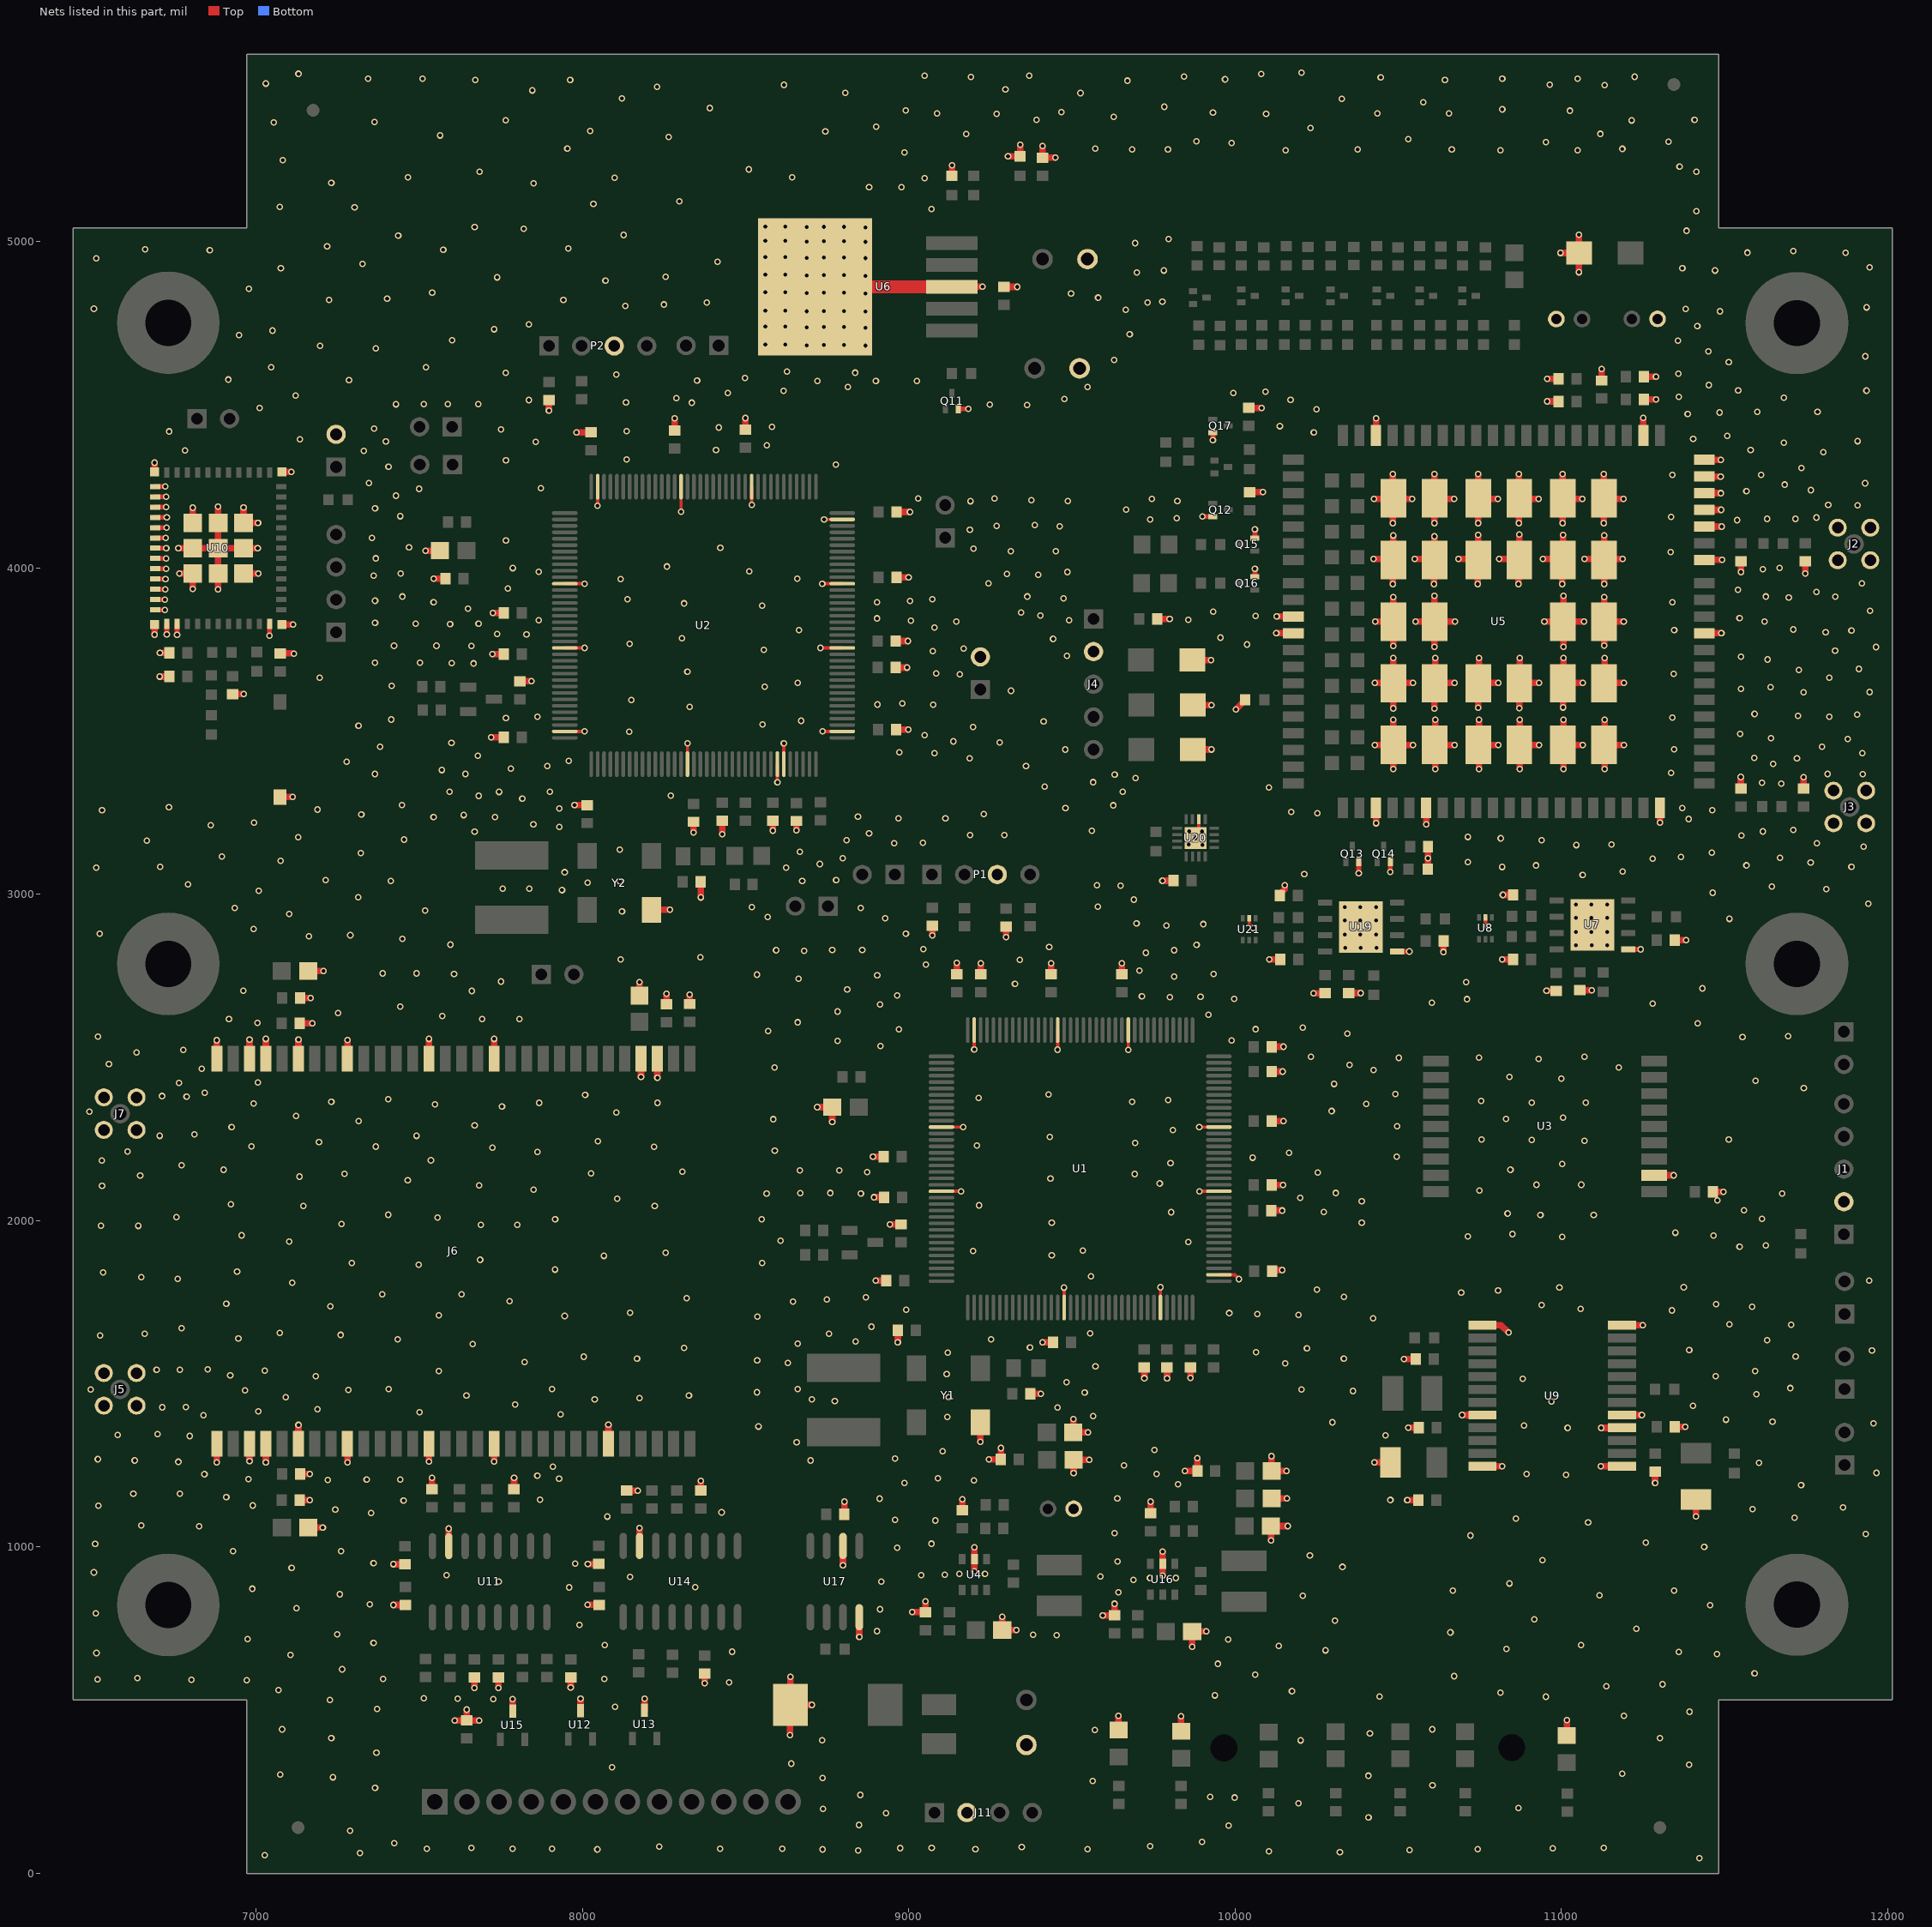
[diagram p0: the nets of this part, all layers, seen from the top]
# Altium PCB MISC86294.PcbDoc (part 4 of 8)
Units mil, origin at the board's own origin, x right, y up, seen from the top; angles counter-clockwise.
Board outline 5574.84 x 5574.84 mil, 4 copper layers (Top, GND02, PWR03, Bottom), stack 23.756 mil thick; 313 components, 311 nets, 1350 pads, 1701 vias.

## Via types
v1: diameter 20, hole 12, Top to Bottom, 1701 vias

## Nets (pads, with @x,y where several pads share a name; then routed paths per layer and width w, separated by ;. In a path a pad name is that pad's centre, name@x,y a point inside that pad or via, vN(x,y) a via of type N, cw(c..) or ccw(c..) an arc to the next point about the centre after c; other vN are vias at no path point) (continued)
GND: C1.1 C2.2 C3.2 C4.2 C5.2 C6.2 C7.2 C8.2 C9.2 C10.2 C11.2 C12.2 C13.2 C14.2 C15.2 C16.2 C17.2 C18.2 C19.1 C20.2 C21.2 C22.2 C23.2 C24.2 C25.2 C26.2 C27.2 C28.2 C29.2 C30.2 C31.2 C32.2 C33.2 C34.2 C35.2 C36.2 C37.2 C40.2 C41.2 C42.2 C43.2 C44.1 C45.1 C46.2 C49.2 C50.2 C51.2 C52.2 C53.1 C55.1 C56.1 C59.2 C60.2 C61.2 C62.2 C64.2 C65.2 C66.2 C67.2 C69.1 C70.1 C74.2 C75.2 C76.2 C77.2 C78.2 C79.2 C80.2 C81.2 C82.2 C83.2 C84.2 C85.2 C86.1 C87.2 C88.2 C89.1 C90.1 C91.1 C92.1 C93.2 C94.2 C95.2 C96.2 C97.2 C98.2 C99.1 C100.1 C101.1 C102.1 C103.1 C104.1 C105.2 C107.2 C110.2 C111.2 C112.2 C113.2 C115.1 C116.1 C117.2 C118.1 C119.1 C120.2 C121.2 C122.1 C123.2 C124.1 C128.2 C129.2 C130.2 C200.1 C201.2 C202.1 C203.2 D1.1 D2.2 D3.2 D4.1 D5.1 D6.1 D7.1 D11.2 J1.2 J2.2 J2.3 J2.4 J2.5 J3.2 J3.3 J3.4 J3.5 J4.2 J5.2 J5.3 J5.4 J5.5 J6.1 J6.3 J6.4 J6.6 J6.9 J6.14 J6.18 J6.25 J6.33 J6.34 J6.43 J6.47 J6.52 J6.55 J6.57 J6.58 J6.60 J7.2 J7.3 J7.4 J7.5 J9.2 J11.2 J23.2 L3.2 P1.3 P2.3 Q11.2 Q12.2 Q13.2 Q14.2 Q15.2 Q16.2 Q17.2 R3.1 R5.1 R11.2 R16.1 R18.1 R20.2 R28.1 R33.1 R61.1 R62.1 R63.1 R85.2 SW1.1 U1.16 U1.31 U1.38 U1.51 U1.61 U1.83 U1.94 U1.107 U1.120 U1.130 U2.16 U2.30 U2.31 U2.38 U2.51 U2.61 U2.71 U2.83 U2.94 U2.107 U2.120 U2.130 U2.143 U3.2 U4.2 U5.8 U5.9 U5.19 U5.22 U5.36 U5.46 U5.48 U5.50 U5.51 U5.52 U5.53 U5.54 U5.56 U5.72 U5.85 U5.86 U5.87 U5.88 U5.89 U5.90 U5.91 U5.92 U5.93 U5.94 U5.95 U5.96 U5.97 U5.98 U5.99 U5.100 U5.101 U5.102 U5.103 U5.104 U5.105 U5.106 U5.107 U5.108 U5.109 U5.110 U5.111 U5.112 U6.3 U6.6 U7.1 U7.9 U8.2 U9.1 U9.8 U9.12 U9.13 U9.16 U9.17 U9.24 U10.1 U10.2 U10.11 U10.36 U10.37 U10.38 U10.39 U10.40 U10.41 U10.42 U10.43 U10.44 U10.45 U10.46 U10.47 U10.48 U10.49 U10.50 U10.51 U10.52 U10.53 U11.15 U12.3 U13.3 U14.15 U15.3 U16.2 U17.2 U17.8 U19.1 U19.9 U20.6 U20.17 U21.2 Y1.2 Y2.2 | length 18190.1
  Top w10: U2.143@7945.42,3499.52 v1(8006.52,3499.52) ; U2.130@7945.42,3755.43 v1(8006.57,3755.43) ; U2.120@7945.42,3952.28 v1(8005.72,3952.28) ; v1(8045.81,4191.19) U2.107@8045.81,4249.52 ; v1(8301.71,4172.71) U2.94@8301.71,4249.52 ; U2.16@8321.4,3399.13 v1(8321.4,3462.6) ; v1(8518.25,4193.25) U2.83@8518.25,4249.52 ; v1(8596.99,3343.01) U2.30@8596.99,3399.13 ; U2.31@8616.67,3399.13 v1(8616.67,3463.32) ; v1(8728.57,3755.43) U2.51@8795.81,3755.43 ; v1(8734.72,3952.28) U2.61@8795.81,3952.28 ; v1(8735.52,3499.52) U2.38@8795.81,3499.52 ; v1(8740.13,4149.13) U2.71@8795.81,4149.13 ; U1.130@9099.8,2090.1 v1(9160.1,2090.1) ; U1.120@9099.8,2286.95 v1(9166.05,2286.95) ; v1(9200.2,2524.8) U1.107@9200.2,2584.2 ; v1(9456.1,2524.1) U1.94@9456.1,2584.2 ; U1.16@9475.79,1733.8 v1(9475.79,1794.79) ; v1(9672.64,2523.36) U1.83@9672.64,2584.2 ; U1.31@9771.06,1733.8 v1(9771.06,1795.94) ; U20.17@9888.99,3203.01 U20.6@9888.99,3230.12 ; v1(9890.05,2286.95) U1.61@9950.2,2286.95 ; v1(9891.1,2090.1) U1.51@9950.2,2090.1 ; U1.38@9950.2,1834.2 9998.8,1834.2 v1(10012,1821) ; U21.2@10043,2926.47 10043,2909 v1(10055,2897)
  Top w12: v1@10767,2909 U8.2@10767,2929.47 ; v1@10773,2904 10772.5,2903.5 10773.5,2903.5 10773.62,2903.62 v1(10774.3,2903.62)
  Top w15: U10.48@6690.09,3872.02 v1(6719.98,3872.02) ; U10.47@6690.09,3903.52 v1(6719.52,3903.52) ; U10.46@6690.09,3935.02 v1(6721.02,3935.02) ; U10.45@6690.09,3966.51 v1(6721.51,3966.51) ; U10.44@6690.09,3998.01 v1(6722.99,3998.01) ; U10.43@6690.09,4029.5 v1(6723.5,4029.5) ; U10.42@6690.09,4061 v1(6724,4061) ; U10.41@6690.09,4092.5 v1(6722.5,4092.5) ; U10.40@6690.09,4123.99 v1(6724.99,4123.99) ; U10.39@6690.09,4155.49 v1(6725.49,4155.49) ; U10.38@6690.09,4186.98 v1(6723.98,4186.98) ; U10.37@6690.09,4218.48 v1(6723.48,4218.48) ; U10.36@6690.09,4249.98 v1(6720.98,4249.98) ; v1(6725.52,3796.52) U10.1@6725.52,3828.72 ; v1(6757.02,3795.02) U10.2@6757.02,3828.72 ; v1(7040.48,3792.48) U10.11@7040.48,3828.72 ; Q11.2@9152.04,4487.7 v1(9182.3,4487.7) ; v1(9900.05,4158.05) Q12.2@9930.93,4158.05 ; v1(9931.93,4392.07) Q17.2@9931.93,4415.6 ; Q16.2@10060.74,3973.48 v1(10060.74,3998.26) ; Q15.2@10060.74,4092.48 v1(10060.74,4118.74) ; v1(10378.92,3065.08) Q13.2@10378.92,3099.74 ; v1(10475.68,3068.32) Q14.2@10475.68,3099.74 ; U19.1@10496.06,2825.03 v1(10534.03,2825.03) ; U7.1@11205.26,2831.5 v1(11242.5,2831.5)
  Top w20: v1(6688.12,3796.12) U10.53@6688.12,3826.75 ; U10.50@6688.12,4295.25 v1(6688.12,4323.12) ; v1(6703.54,3667.46) C102.1@6733.79,3667.46 ; v1(6704.46,3740.46) C103.1@6733.79,3740.46 ; v1(6760.99,4060.99) U10.49@6805.24,4060.99 ; v1(6764.24,3983.24) U10.49@6805.24,3983.24 v1(6805.24,3935.76) ; U10.49@6805.24,4138.75 v1(6805.24,4185.24) ; U10.49@6828.01,4060.99 U10.49@6883,4060.99 ; v1(6879.01,1258.99) J6.1@6879.01,1315.83 ; J6.60@6879.01,2496.94 v1(6879.01,2552.99) ; v1(6883,3935) U10.49@6883,3983.24 ; U10.49@6883,3998 U10.49@6883,4060.99 ; U10.49@6883,4113 U10.49@6883,4060.99 ; U10.49@6883,4138.75 v1(6883,4188) ; C104.1@6927.54,3613.79 v1(6961.79,3613.79) ; U10.49@6942.99,4060.99 U10.49@6883,4060.99 ; U10.49@6960.76,3983.24 v1(7006.24,3983.24) ; U10.49@6960.76,4060.99 v1(7003.99,4060.99) ; v1(6960.76,4185.76) U10.49@6960.76,4138.75 v1(7005.25,4138.75) ; v1(6979.01,1263.01) J6.3@6979.01,1315.83 ; J6.58@6979.01,2496.94 v1(6979.01,2555.01) ; v1(7029.01,1259.01) J6.4@7029.01,1315.83 ; J6.57@7029.01,2496.94 v1(7029.01,2557.01) ; SW1.1@7072.43,3298.37 v1(7111.37,3298.37) ; C105.2@7072.68,3738.82 v1@7113.18,3738.82 ; U10.52@7077.88,3826.75 v1(7112.75,3826.75) ; U10.51@7077.88,4295.25 v1(7106.75,4295.25) ; J6.6@7129.01,1315.83 v1(7129.01,1373.99) ; J6.55@7129.01,2496.94 v1(7129.01,2554.99) ; C90.1@7132.87,2604.56 v1(7171.56,2604.56) ; C88.2@7133.25,1143.3 v1(7163.7,1143.3) ; C87.2@7133.55,1223.2 v1(7163.8,1223.2) ; C89.1@7134.24,2682.56 v1(7166.56,2682.56) ; C91.1@7159.09,2765.45 v1(7205.55,2765.45) ; C86.1@7159.25,1059.3 v1(7203.7,1059.3) ; v1(7279.01,1259.01) J6.9@7279.01,1315.83 ; J6.52@7279.01,2496.94 v1(7279.01,2554.01) ; v1(7419.76,822.24) C110.2@7457.16,822.24 ; v1(7420.14,947.14) C107.2@7455.89,947.14 ; v1(7518.53,4053.47) C28.2@7562.55,4053.47 ; v1(7529.01,1262.01) J6.14@7529.01,1315.83 ; J6.47@7529.01,2496.94 v1(7529.01,2557.01) ; C115.1@7538.64,1177.45 v1(7538.64,1211.36) ; v1(7543.45,3967.55) C22.2@7579.14,3967.55 ; U11.15@7590.02,1002.38 v1(7590.02,1056.02) ; v1(7607.75,468.25) L3.2@7644.59,468.25 ; v1(7644.59,501.59) L3.2@7644.59,468.25 ; v1(7667.93,567.93) C113.2@7667.93,600.24 ; v1(7683.25,468.25) L3.2@7644.59,468.25 ; v1(7720,3481) C25.2@7758.14,3481 ; v1(7723.7,3736.7) C23.2@7758.14,3736.7 ; v1(7725.15,3862.85) C24.2@7758.14,3862.85 ; v1(7729.01,1261.99) J6.18@7729.01,1315.83 ; J6.43@7729.01,2496.94 v1(7729.01,2556.99) ; v1(7741.82,568.18) C121.2@7741.82,600.24 ; U15.3@7785.4,496.71 v1(7785.4,533.6) ; C116.1@7789.89,1177.45 v1(7789.89,1211.89) ; R16.1@7807.89,3653.25 v1(7843.25,3653.25) ; v1(7896.51,4482.51) R20.2@7896.51,4515.6 ; v1(7963.48,569.48) C120.2@7963.48,600.24 ; v1(7975.32,3273.68) C203.2@8014.05,3273.68 ; v1(7981.08,4415.92) C34.2@8026.08,4415.92 ; U12.3@7993.6,498.71 v1(7993.6,535.4) ; v1(8015.66,822.34) C112.2@8051.36,822.34 ; v1(8015.94,947.94) C111.2@8049.91,947.94 ; J6.25@8079.01,1315.83 v1(8079.01,1374.99) ; C118.1@8134.38,1172.45 v1(8169.55,1172.45) ; C101.1@8174.55,2690.09 v1(8174.55,2730.55) ; U14.15@8174.68,1003.16 v1(8174.68,1058.32) ; v1(8179.01,2440.99) J6.34@8179.01,2496.94 ; U13.3@8189.75,498.96 v1(8189.75,535.25) ; Y2.2@8209.69,2953.06 v1(8268.06,2953.06) ; v1(8229.01,2438.01) J6.33@8229.01,2496.94 ; C100.1@8257.44,2663.75 v1(8257.44,2695.56) ; C27.2@8281.83,4421.48 v1(8281.83,4459.17) ; C99.1@8328.44,2663.99 v1(8328.44,2692.44) ; v1(8339.7,3189.3) C29.2@8339.7,3222.52 ; C119.1@8361.88,1172.45 v1(8361.88,1202.88) ; v1(8362.29,2990.71) C202.1@8362.29,3026 ; v1(8374.53,582.53) C117.2@8374.53,612.24 ; v1(8428.25,3184.25) C19.1@8428.25,3224.63 ; C31.2@8498.76,4424.48 v1(8498.76,4459.77) ; v1(8582.6,3195.6) C21.2@8582.6,3226.14 ; v1(8636,423) D1.1@8636,465 ; v1(8636.87,602.13) D1.1@8636.87,516 v1(8703,516) ; v1(8655.74,3196.26) C20.2@8655.74,3225.14 ; v1(8719,2348) C12.2@8765.1,2348 v1(8765.1,2303.1) ; v1(8798,944) U17.2@8798,1003 ; C124.1@8802.11,1100.18 v1(8802.11,1138.89) ; v1(8848,724) U17.8@8848,784.7 ; v1(8889.94,2196.06) C14.2@8922.52,2196.06 ; v1(8893.17,2071.83) C13.2@8924.52,2071.83 ; v1(8898,1816) C11.2@8930.14,1816 ; v1(8941.5,1988.5) R3.1@8975.89,1988.5 ; R18.1@8959.03,3695.11 v1(8994.11,3695.11) ; C30.2@8959.48,3776.47 v1(8996.53,3776.47) ; C26.2@8960.48,3505.41 8997.59,3505.41 v1(8998,3505) ; C33.2@8961.77,4172.02 v1(9003.02,4172.02) ; C32.2@8962.48,3972 v1(8999,3972) ; v1(8965.99,1627.01) C201.2@8965.99,1664.16 ; v1(9010.25,800.25) C45.1@9050.89,800.25 v1(9050.89,832.89) ; v1(9071.89,2874.11) R11.2@9071.89,2903.92 ; U6.3@9132.07,4862.15 v1(9226.15,4862.15) ; R63.1@9132.17,5202.48 v1(9132.17,5234.83) ; C15.2@9147.3,2755.48 v1(9147.3,2790.3) ; R28.1@9163.89,1112.25 v1(9163.89,1145.89) ; v1(9201,925) U4.2@9201,962.24 v1(9201,999) ; v1(9219.62,1322.38) Y1.2@9219.62,1381.7 ; C2.2@9220.11,2755.48 v1(9220.11,2789.11) ; v1(9245.11,1268.11) C41.2@9282.14,1268.11 v1(9282.14,1303.14) ; v1(9286.2,785.8) C44.1@9286.2,745 v1(9329,745) ; C75.2@9291.05,4862.01 v1(9331.99,4862.01) ; v1(9298,2869) C1.1@9298,2901.75 ; v1(9303.84,5262.16) R61.1@9341.05,5262.16 v1(9341.05,5298.05) ; C200.1@9372.08,1469.16 v1(9404.16,1469.16) ; v1(9410,1627) C18.2@9441.52,1627 ; v1(9410.05,5293.95) C77.2@9410.05,5257.96 v1(9448.96,5257.96) ; C16.2@9435.53,2755.48 v1(9435.53,2788.53) ; v1(9503.9,1391.9) C40.2@9503.9,1351 v1(9549,1351) ; v1(9504.9,1226.1) C42.2@9504.9,1267 v1(9553,1267) ; v1(9594.32,790.32) C92.1@9630.01,790.32 v1(9630.01,825.99) ; D11.2@9642.55,438.8 v1(9642.55,482.45) ; C17.2@9652.76,2755.48 v1(9652.76,2788.76) ; v1(9721.74,1517.26) C6.2@9721.74,1550.14 ; R33.1@9740.89,1103.25 v1(9740.89,1138.89) ; C62.2@9760.83,3844.65 v1(9799.35,3844.65) ; v1(9777.11,3041.89) C122.1@9811.75,3041.89 ; v1(9778,912) U16.2@9778,948.24 v1(9778,986) ; v1(9791.37,1516.37) C5.2@9791.37,1550.14 ; D3.2@9834.55,434.8 v1(9834.55,481.55) ; v1(9846.11,1233.11) C50.2@9884.14,1233.11 v1(9884.14,1271.86) ; v1(9862.63,1518.37) C4.2@9862.63,1550.14 ; v1(9868.2,694.2) C53.1@9868.2,741 v1(9912,741) ; D5.1@9868.79,3718.07 v1(9926.07,3718.07) ; D6.1@9869.79,3444.07 v1(9927.93,3444.07) ; D7.1@9869.79,3580.07 v1(9927.93,3580.07) ; v1(10002,3567.34) R62.1@10030.74,3596.07 ; C81.2@10041.5,4490.93 v1(10080.93,4490.93) ; C78.2@10044.94,4232.93 v1(10084.93,4232.93) ; v1(10104.44,2800.56) C129.2@10138.47,2800.56 ; v1(10109.9,1020.1) C51.2@10109.9,1064 v1(10161,1064) ; R5.1@10111.25,2031.11 v1(10143.89,2031.11) ; C8.2@10111.86,2109.45 v1(10146.55,2109.45) ; C9.2@10111.86,2305.3 v1(10148.7,2305.3) ; C3.2@10111.86,2457 v1(10146,2457) ; C10.2@10111.86,2533.15 v1(10147.85,2533.15) ; C49.2@10111.9,1149 v1(10159,1149) ; v1(10111.9,1278.1) C52.2@10111.9,1233 v1(10157,1233) ; C7.2@10112.86,1848.6 v1(10144.4,1848.6) ; v1(10126.42,3800.57) U5.9@10178.08,3800.57 ; v1(10127.76,3851.76) U5.8@10178.08,3851.76 ; C123.2@10137.31,2996.24 10137.31,3001.31 10152,3016 v1(10152,3028) ; v1(10239.86,2697.14) C93.2@10275.89,2697.14 ; C128.2@10347.55,2697.47 v1(10384.53,2697.47) ; v1(10424.06,4027.94) 10483.84,4027.94 v1(10483.84,3951.16) ; v1(10425.94,4212.06) U5.108@10483.16,4212.06 ; v1(10427,1259) C37.2@10475.99,1259 ; v1(10427.94,3458.06) U5.112@10485.16,3458.06 ; v1(10427.94,3648.06) U5.111@10485.16,3648.06 ; v1(10429,3836.01) U5.110@10485.16,3836.01 ; v1(10432.01,3218.01) U5.19@10432.01,3265.13 ; U5.72@10432.01,4406.86 v1(10432.01,4458.99) ; v1(10483.16,4137.84) U5.108@10483.16,4212.06 ; v1(10483.16,4288.84) U5.108@10483.16,4212.06 ; v1(10485.16,3383.84) U5.112@10485.16,3458.06 ; v1(10485.16,3534.84) U5.112@10485.16,3458.06 ; v1(10485.16,3570.16) U5.111@10485.16,3647.02 ; v1(10485.16,3724.84) U5.111@10485.16,3648.06 ; v1(10485.16,3761.16) U5.110@10485.16,3836.01 ; v1(10485.16,3911.16) U5.110@10485.16,3836.01 ; U5.109@10485.16,4024.98 v1(10485.16,4099.84) ; v1(10517.89,1576.11) C96.2@10554.14,1576.11 ; v1(10527.5,1143.5) C98.2@10561.14,1143.5 ; v1(10530.98,1365.98) C94.2@10562.31,1365.98 ; v1(10542.94,4212.06) U5.108@10483.16,4212.06 ; v1(10544.94,3458.06) U5.112@10485.16,3458.06 ; v1(10544.94,3648.06) U5.111@10485.16,3648.06 ; v1(10550.06,4027.94) 10609.84,4027.94 v1(10609.84,3951.16) ; v1(10553,3836.01) U5.105@10611.15,3836.01 ; v1(10585.55,3214.55) U5.22@10585.55,3265.13 ; R85.2@10590.67,3077.13 v1@10590.67,3108.67 ; v1(10591.13,3110.87) C79.2@10591.13,3146.93 ; v1(10611.14,3569.86) U5.106@10611.14,3647.02 ; v1(10611.15,3759.15) U5.105@10611.15,3836.01 ; v1(10611.15,3914.85) U5.105@10611.15,3836.01 ; U5.104@10611.14,4024.98 v1(10611.14,4097.14) ; v1(10611.16,4137.84) U5.103@10611.16,4212.06 ; v1(10611.16,4288.84) U5.103@10611.16,4212.06 ; v1(10613.16,3383.84) U5.107@10613.16,3458.06 ; v1(10613.16,3534.84) U5.107@10613.16,3458.06 ; v1(10613.16,3724.84) 10613.16,3648.06 v1(10672.94,3648.06) ; v1(10638.53,2823.53) C130.2@10638.53,2856.97 ; v1(10670.94,4212.06) U5.103@10611.16,4212.06 ; v1(10672.94,3458.06) U5.107@10613.16,3458.06 ; v1(10674,3836.01) U5.105@10611.15,3836.01 ; v1(10684.06,4027.94) 10743.84,4027.94 v1(10743.84,3951.16) ; v1(10695.64,1404.36) U9.8@10758.02,1404.36 ; v1(10745,3572) U5.101@10745,3647.02 ; U5.100@10745,4024.98 v1(10745,4102) ; v1(10745.16,4137.84) U5.99@10745.16,4212.06 ; v1(10745.16,4288.84) U5.99@10745.16,4212.06 ; v1(10747.16,3383.84) U5.102@10747.16,3458.06 ; v1(10747.16,3534.84) U5.102@10747.16,3458.06 ; v1(10747.16,3724.84) 10747.16,3648.06 v1(10806.94,3648.06) ; U9.12@10758.02,1246.88 v1(10818.12,1246.88) ; U9.1@10758.02,1679.95 10815.05,1679.95 v1(10838,1657) ; v1(10804.94,4212.06) U5.99@10745.16,4212.06 ; v1(10806.94,3458.06) U5.102@10747.16,3458.06 ; v1(10809.06,4027.94) 10868.84,4027.94 v1(10868.84,3951.16) ; v1(10818.03,2801.03) C84.2@10851.47,2801.03 ; v1(10820.55,2998.45) C82.2@10852.47,2998.45 ; v1(10870.16,4137.84) U5.95@10870.16,4212.06 ; v1(10870.16,4288.84) U5.95@10870.16,4212.06 ; v1(10870.99,3571.01) U5.97@10870.99,3647.02 ; U5.96@10870.99,4024.98 v1(10870.99,4102.99) ; v1(10872.16,3383.84) U5.98@10872.16,3458.06 ; v1(10872.16,3534.84) U5.98@10872.16,3458.06 ; v1(10872.16,3724.84) 10872.16,3648.06 v1(10931.94,3648.06) ; v1(10929.94,4212.06) U5.95@10870.16,4212.06 ; v1(10931.94,3458.06) U5.98@10872.16,3458.06 ; v1(10943.06,4027.94) 11002.84,4027.94 v1(11002.84,3951.16) ; v1(10948,3836.01) U5.92@11006.15,3836.01 ; v1(10954.47,2704.47) C83.2@10984.44,2704.47 ; v1(10956.73,4580.27) C66.2@10991.17,4580.27 ; v1(10956.97,4511.03) C67.2@10991.17,4511.03 ; v1(10997.07,4965.93) D4.1@11054.21,4965.93 ; v1(11004.16,4137.84) U5.90@11004.16,4212.06 ; v1(11004.16,4288.84) U5.90@11004.16,4212.06 ; v1(11004.85,3572.85) U5.93@11004.85,3647.02 ; U5.91@11004.85,4024.98 v1(11004.85,4101.85) ; v1(11006.16,3383.84) U5.94@11006.16,3458.06 ; v1(11006.16,3534.84) U5.94@11006.16,3458.06 ; v1(11006.16,3724.84) 11006.16,3648.06 v1(11065.94,3648.06) ; v1(11006.15,3759.15) U5.92@11006.15,3836.01 ; v1(11006.15,3914.85) U5.92@11006.15,3836.01 ; D2.2@11016.55,421.8 v1(11016.55,469.55) ; v1(11054.21,4906.79) D4.1@11054.21,4965.93 ; v1(11054.21,5021.79) D4.1@11054.21,4965.93 ; C80.2@11055.89,2706.14 v1(11093.14,2706.14) ; v1(11063.94,4212.06) U5.90@11004.16,4212.06 ; v1(11065.94,3458.06) U5.94@11006.16,3458.06 ; v1(11069,3836.01) U5.92@11006.15,3836.01 ; v1(11071.06,4027.94) U5.86@11130.84,4027.94 ; v1(11121.12,1246.88) U9.13@11185.98,1246.88 ; v1(11122.01,1364.99) U9.16@11185.98,1364.99 ; C61.2@11123.35,4574.83 v1(11123.35,4610.35) ; v1(11130.16,4137.84) U5.85@11130.16,4212.06 ; v1(11130.16,4288.84) U5.85@11130.16,4212.06 ; v1(11130.83,3762.17) U5.87@11130.83,3836.01 ; v1(11130.83,3910.83) U5.87@11130.83,3836.01 ; v1(11130.84,3951.16) U5.86@11130.84,4027.94 ; U5.86@11130.83,4024.98 v1(11130.83,4100.83) ; v1(11132.16,3383.84) U5.89@11132.16,3458.06 ; v1(11132.16,3534.84) U5.89@11132.16,3458.06 ; v1(11132.16,3724.84) 11132.16,3648.06 v1(11191.94,3648.06) ; U9.17@11185.98,1404.36 v1(11246.36,1404.36) ; U9.24@11185.98,1679.95 v1(11249.95,1679.95) ; v1(11188.06,4027.94) U5.86@11130.84,4027.94 ; v1(11189.94,4212.06) U5.85@11130.16,4212.06 ; v1(11191,3836.01) U5.87@11130.83,3836.01 ; v1(11191.94,3458.06) U5.89@11132.16,3458.06 ; U5.56@11250.91,4406.86 v1(11250.91,4460.91) ; C60.2@11252.83,4516.65 v1(11290.65,4516.65) ; C65.2@11252.83,4586.73 v1(11289.73,4586.73) ; U3.2@11284.65,2139 v1(11344,2139) ; v1(11287.09,1196.09) C95.2@11287.09,1231.15 ; v1(11302.09,3219.91) U5.36@11302.09,3265.13 ; C97.2@11347.12,1367.7 v1(11379.7,1367.7) ; C85.2@11347.86,2859.89 v1(11381.89,2859.89) ; v1(11412,1094) C36.2@11412,1144.99 ; U5.46@11437.92,3800.57 v1(11490.58,3800.57) ; U5.48@11437.92,4024.98 v1(11492.99,4024.98) ; U5.50@11437.92,4127.35 v1(11491.34,4127.35) ; U5.51@11437.92,4178.52 v1(11489.48,4178.52) ; U5.52@11437.92,4229.7 v1(11488.3,4229.7) ; U5.53@11437.92,4280.89 v1(11488.11,4280.89) ; U5.54@11437.92,4332.06 v1(11488.93,4332.06) ; C35.2@11463.86,2088.89 v1(11496.89,2088.89) ; C70.1@11549.89,3324.25 v1(11549.89,3359.89) ; v1(11549.98,3988.02) C56.1@11549.98,4021.43 ; C69.1@11742.19,3324.18 v1(11742.19,3359.19) ; v1(11748.08,3983.92) C55.1@11748.08,4020.43
  Top w40: U6.6@8872.85,4862.15 U6.3@9132.07,4862.15
  Bottom w12: v1(10774.3,2903.62) v1@10774.3,2903.7